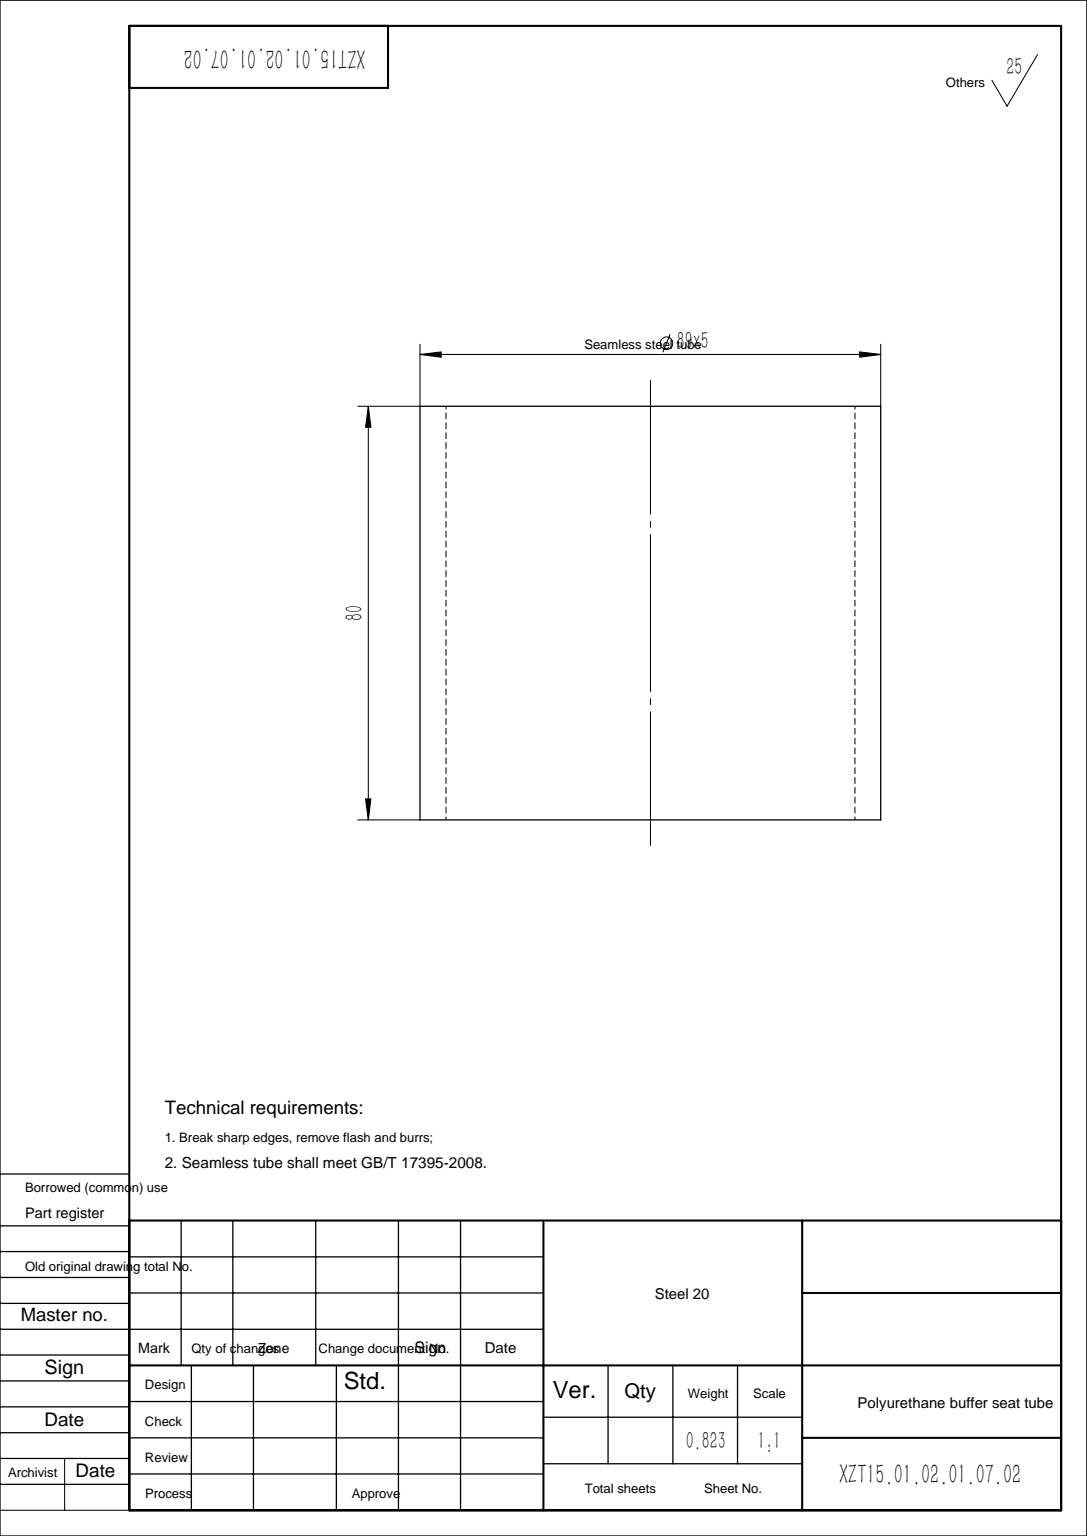
from build123d import *

# Parameters (mm, degrees)
SKETCH1_R           = 44.5
SKETCH1_R_2         = 39.5
BOSS_EXTRUDE1_DEPTH = 80


with BuildPart() as part:
    # Sketch1 → Boss-Extrude1 (new body)
    with BuildSketch(Plane(origin=(0, 0, 0), x_dir=(1, 0, 0), z_dir=(0, 1, 0))):
        with Locations(Location((0, 0, 0), (0, 0, 270))):
            Circle(SKETCH1_R)
        with Locations(Location((0, 0, 0), (0, 0, 270))):
            Circle(SKETCH1_R_2, mode=Mode.SUBTRACT)
    extrude(amount=BOSS_EXTRUDE1_DEPTH)


solid = part.part
